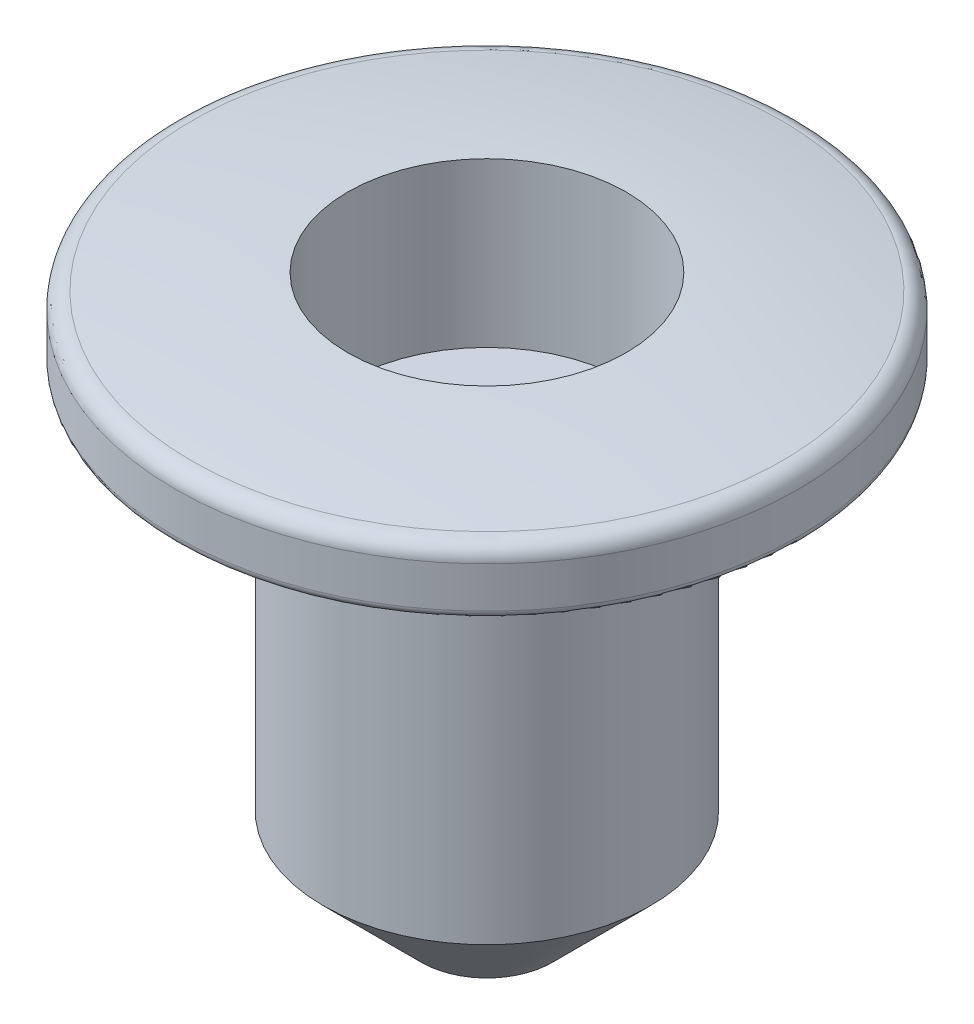
SolidWorks part; units mm, degrees
ref_plane "Front Plane" through (0, 0, 0) normal (0, 0, 1) x (1, 0, 0)
ref_plane "Top Plane" through (0, 0, 0) normal (0, 1, 0) x (1, 0, 0)
ref_plane "Right Plane" through (0, 0, 0) normal (1, 0, 0) x (0, 0, -1)
other "Configuration Table"
sketch "Sketch1" plane through (0, 0, 0) normal (0, 0, 1) x (1, 0, 0)
  line L0 (0, 0) -> (0, -20)
  line L1 (0, -20) -> (-3.5, -20)
  line L2 (-3.5, -20) -> (-10, -13.5)
  line L3 (-10, -13.5) -> (-10, 6)
  line L4 (-14, 10) -> (-18.5, 10)
  line L5 (-19, 10.5) -> (-19, 13)
  line L6 (-18, 14) -> (0, 14) construction
  line L7 (0, 14) -> (0, 0)
  line L8 (0, 15) -> (0, 14)
  line L9 (0, 15) -> (-2, 15)
  line L10 (-0.5791, 15) -> (0, 14.5764)
  line L11 (0, -18.5) -> (-2.8787, -18.5)
  line L12 (-2.8787, -18.5) -> (-8.5, -12.8787)
  line L13 (-8.5, -12.8787) -> (-8.5, 3.5)
  line L14 (-8.5, -12.8787) -> (-8.5, 6) construction
  line L15 (-8.5, 5) -> (-5.5, 5)
  line L16 (-5.5, 5) -> (-5.5, 3.5)
  line L17 (-5.5, 3.5) -> (-8.5, 3.5)
  line L18 (-8.5, 5) -> (-8.5, 14.9772)
  arc A0 (-10, 6) -> (-14, 10) centre (-14, 6) ccw
  arc A1 (-19, 13) -> (-18, 14) centre (-18, 13) cw
  arc A2 (-2, 15) -> (-18, 14) centre (-4.9664, -66.0377) ccw
  arc A3 (-18.5, 10) -> (-19, 10.5) centre (-18.5, 10.5) cw
  point P10 (-19, 14)
  point P22 (-19, 10)
  dimension "D7" = 4
  dimension "D10" = 1
  dimension "D11" = 1
  dimension "D12" = 2
  dimension "D13" = 81.092
  dimension "D14" = 0.5
  dimension "D1" = 10
  dimension "D2" = 3.5
  dimension "D3" = 45
  dimension "D4" = 6.5
  dimension "D5" = 20
  dimension "D6" = 19
  dimension "D8" = 30
  dimension "D9" = 4
  dimension "D15" = 1.5
  dimension "D16" = 3
  dimension "D17" = 25
  dimension "D18" = 1.5
revolve "Revolve1" add sketch "Sketch1" angle 360 about L7
sketch "Sketch3" plane through (0, -20, 0) normal (0, -1, 0) x (1, 0, 0)
  circle A0 centre (0, 0) radius 2.75
  dimension "D1" = 5.5
extrude "Cut-Extrude1" cut sketch "Sketch3" against normal blind 10
sketch "Sketch4" plane through (0, -20, 0) normal (0, -1, 0) x (1, 0, 0)
  circle A0 centre (0, 0) radius 4
  dimension "D1" = 8
extrude "Cut-Extrude2" cut sketch "Sketch4" against normal blind 10
